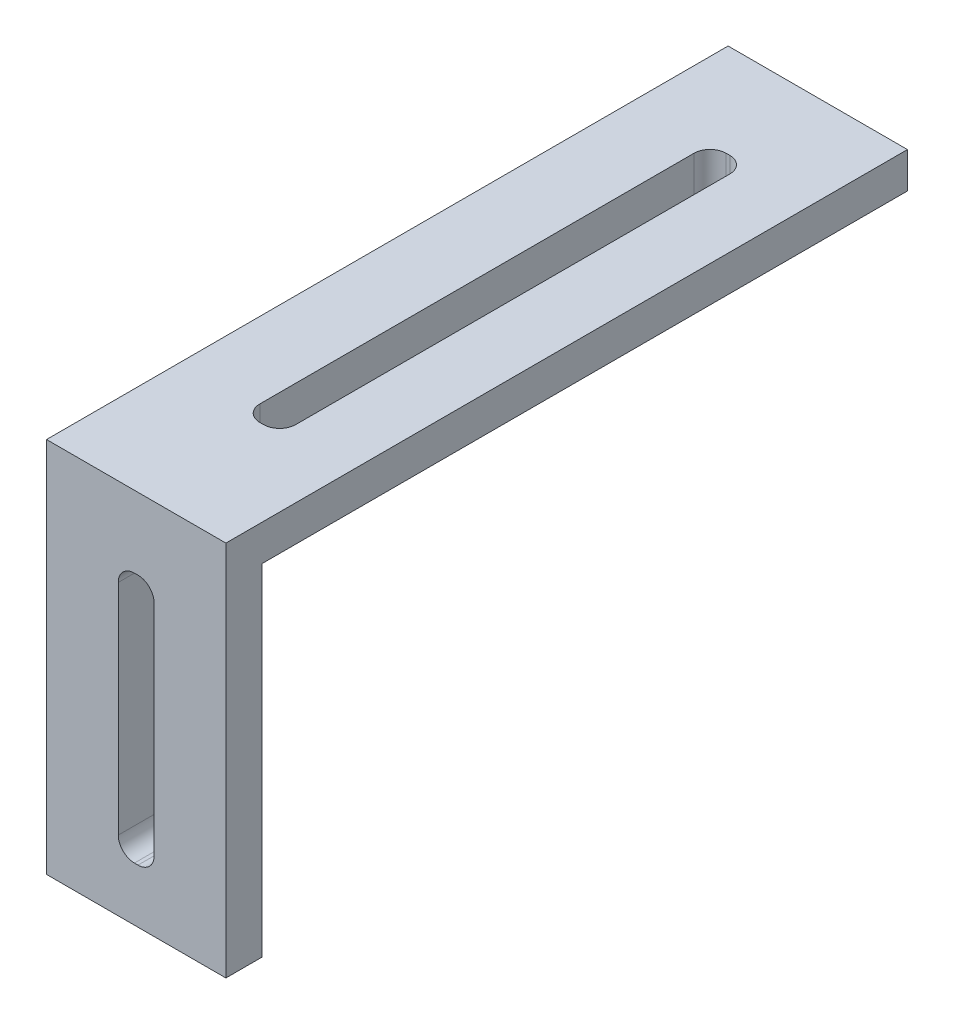
SolidWorks part; units mm, degrees
material "PVC Rigid"
ref_plane "Front Plane" through (0, 0, 0) normal (0, 0, 1) x (1, 0, 0)
ref_plane "Top Plane" through (0, 0, 0) normal (0, 1, 0) x (1, 0, 0)
ref_plane "Right Plane" through (0, 0, 0) normal (1, 0, 0) x (0, 0, -1)
sketch "Sketch1" plane through (0, 0, 0) normal (0, 0, 1) x (1, 0, 0)
  line L1 (25, -50) -> (-25, -50)
  line L2 (25, -50) -> (25, 50)
  line L3 (25, 50) -> (-25, 50)
  line L4 (-25, -50) -> (-25, 50)
  line L5 (25, -50) -> (-25, 50) construction
  line L6 (25, 50) -> (-25, -50) construction
  point P0 (0, 0)
  dimension "D1" = 50
  dimension "D2" = 100
extrude "Boss-Extrude1" add sketch "Sketch1" along normal blind 10
sketch "Sketch2" plane through (0, 0, 10) normal (0, 0, 1) x (1, 0, 0)
  line L1 (0.5, -35) -> (-0.5, -35)
  line L2 (5, -30.5) -> (5, 30.5)
  line L3 (0.5, 35) -> (-0.5, 35)
  line L4 (-5, -30.5) -> (-5, 30.5)
  line L5 (5, -35) -> (-5, 35) construction
  line L6 (5, 35) -> (-5, -35) construction
  arc A0 (-0.5, -35) -> (-5, -30.5) centre (-0.5, -30.5) cw
  arc A1 (0.5, -35) -> (5, -30.5) centre (0.5, -30.5) ccw
  arc A2 (5, 30.5) -> (0.5, 35) centre (0.5, 30.5) ccw
  arc A3 (-0.5, 35) -> (-5, 30.5) centre (-0.5, 30.5) ccw
  point P0 (0, 0)
  dimension "D3" = 4.5
  dimension "D1" = 10
  dimension "D2" = 70
extrude "Cut-Extrude1" cut sketch "Sketch2" against normal blind 10
sketch "Sketch3" plane through (0, 0, 0) normal (0, 0, -1) x (-1, 0, 0)
  line L0 (-25, 50) -> (25, 50) construction
  line L1 (25, 45) -> (-25, 45)
  line L2 (25, 45) -> (25, 55)
  line L3 (25, 55) -> (-25, 55)
  line L4 (-25, 45) -> (-25, 55)
  line L5 (25, 45) -> (-25, 55) construction
  line L6 (25, 55) -> (-25, 45) construction
  line L7 (-25, -50) -> (-25, 50) construction
  line L8 (25, 50) -> (25, -50) construction
  point P0 (0, 50)
  dimension "D1" = 10
extrude "Boss-Extrude2" add sketch "Sketch3" along normal blind 180 and the other way blind 10
sketch "Sketch4" plane through (0, 45, 0) normal (0, -1, 0) x (1, 0, 0)
  line L1 (1.6349, -153.8429) -> (0.6349, -153.8429)
  line L2 (6.1349, -149.3429) -> (6.1349, -28.3429)
  line L3 (1.6349, -23.8429) -> (0.6349, -23.8429)
  line L4 (-3.8651, -149.3429) -> (-3.8651, -28.3429)
  line L5 (6.1349, -153.8429) -> (-3.8651, -23.8429) construction
  line L6 (6.1349, -23.8429) -> (-3.8651, -153.8429) construction
  arc A0 (1.6349, -153.8429) -> (6.1349, -149.3429) centre (1.6349, -149.3429) ccw
  arc A1 (0.6349, -153.8429) -> (-3.8651, -149.3429) centre (0.6349, -149.3429) cw
  arc A2 (0.6349, -23.8429) -> (-3.8651, -28.3429) centre (0.6349, -28.3429) ccw
  arc A3 (6.1349, -28.3429) -> (1.6349, -23.8429) centre (1.6349, -28.3429) ccw
  point P0 (1.1349, -88.8429)
  dimension "D3" = 4.5
  dimension "D1" = 10
  dimension "D2" = 130
extrude "Cut-Extrude2" cut sketch "Sketch4" against normal blind 180
